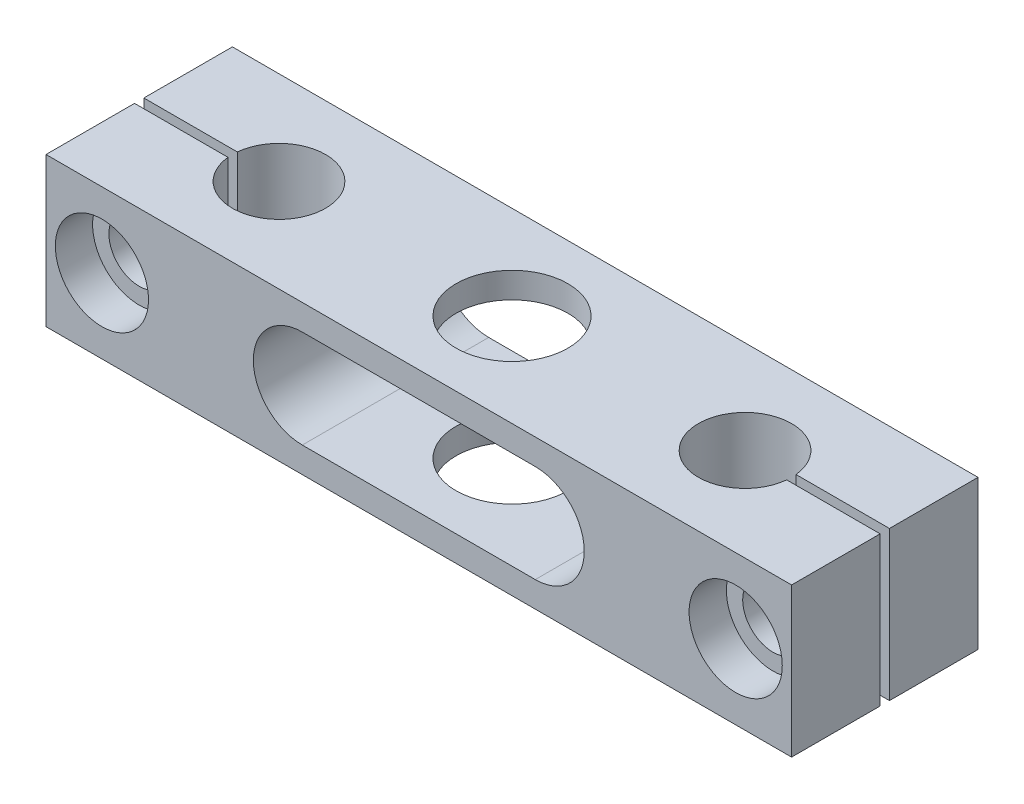
from build123d import *

# Parameters (mm, degrees)
SKETCH1_W                  = 80
SKETCH1_H                  = 16
BOSS_EXTRUDE1_DEPTH        = 20
SKETCH2_R                  = 5
CUT_EXTRUDE1_DEPTH         = 20
SKETCH4_R                  = 6
CUT_EXTRUDE2_DEPTH         = 16.5
SKETCH5_W                  = 29.106163607
SKETCH5_H                  = 1
SKETCH5_W_2                = 37.036491662
CUT_EXTRUDE3_DEPTH         = 30
M6_TAPPED_HOLE1_AT_2_COUNT = 2
M6_TAPPED_HOLE1_AT_2_PITCH = 68
SKETCH8_R                  = 3.25
CUT_EXTRUDE4_DEPTH         = 30
SKETCH9_R                  = 5
CUT_EXTRUDE5_DEPTH         = 4


with BuildPart() as part:
    # Sketch1 → Boss-Extrude1 (new body)
    with BuildSketch(Plane.XY):
        with Locations((9.337676654, 6.4605919)):
            Rectangle(SKETCH1_W, SKETCH1_H)
        with BuildLine():
            Line((-3.162323346, 11.7105919), (21.837676654, 11.7105919))
            ThreePointArc((21.837676654, 11.7105919), (27.087676654, 6.4605919), (21.837676654, 1.2105919))
            Line((21.837676654, 1.2105919), (-3.162323346, 1.2105919))
            ThreePointArc((-3.162323346, 1.2105919), (-8.412323346, 6.4605919), (-3.162323346, 11.7105919))
        make_face(mode=Mode.SUBTRACT)
    extrude(amount=BOSS_EXTRUDE1_DEPTH)

    # Sketch2 → Cut-Extrude1 (cut)
    with BuildSketch(Plane.XZ.offset(1.5394081)):
        with Locations(Location((34.337676654, 10, 0), (0, 0, 270))):
            Circle(SKETCH2_R)
        with Locations(Location((-15.662323346, 10, 0), (0, 0, 270))):
            Circle(SKETCH2_R)
    extrude(amount=-CUT_EXTRUDE1_DEPTH, mode=Mode.SUBTRACT)

    # Sketch4 → Cut-Extrude2 (cut, symmetric)
    with BuildSketch(Plane.XZ.offset(-11.7105919)):
        with Locations(Location((9.337676654, 10, 0), (0, 0, 270))):
            Circle(SKETCH4_R)
    extrude(amount=CUT_EXTRUDE2_DEPTH, both=True, mode=Mode.SUBTRACT)

    # Sketch5 → Cut-Extrude3 (cut)
    with BuildSketch(Plane.XZ.offset(1.5394081)):
        with Locations((48.890758457, 10)):
            Rectangle(SKETCH5_W, SKETCH5_H)
        with Locations((-34.180569177, 10)):
            Rectangle(SKETCH5_W_2, SKETCH5_H)
    extrude(amount=-CUT_EXTRUDE3_DEPTH, mode=Mode.SUBTRACT)

    # Sketch6 → M6 Tapped Hole1 (revolve, cut)
    with BuildSketch(Plane(origin=(43.337676654, 6.4605919, 9.5), x_dir=(0, -1, 0), z_dir=(1, 0, 0))):
        Polygon((0, 0), (0, 18.502151548), (2.5, 17), (2.5, 0), align=None)
    m6_tapped_hole1 = revolve(axis=Axis((43.337676654, 6.4605919, 15.85), (0, 0, -1)), mode=Mode.SUBTRACT)

    # M6 Tapped Hole1 at 2: M6 Tapped Hole1 ×2
    with Locations(*[(-i * M6_TAPPED_HOLE1_AT_2_PITCH, 0, 0) for i in range(1, M6_TAPPED_HOLE1_AT_2_COUNT)]):
        add(m6_tapped_hole1, mode=Mode.SUBTRACT)

    # Sketch8 → Cut-Extrude4 (cut)
    with BuildSketch(Plane(origin=(0, 0, 10.5), x_dir=(-1, 0, 0), z_dir=(0, 0, -1))):
        with Locations((24.662323346, 6.4605919)):
            Circle(SKETCH8_R)
        with Locations((-43.337676654, 6.4605919)):
            Circle(SKETCH8_R)
    extrude(amount=-CUT_EXTRUDE4_DEPTH, mode=Mode.SUBTRACT)

    # Sketch9 → Cut-Extrude5 (cut)
    with BuildSketch(Plane.XY.offset(20)):
        with Locations((43.337676654, 6.4605919)):
            Circle(SKETCH9_R)
        with Locations((-24.662323346, 6.4605919)):
            Circle(SKETCH9_R)
    extrude(amount=-CUT_EXTRUDE5_DEPTH, mode=Mode.SUBTRACT)


solid = part.part
